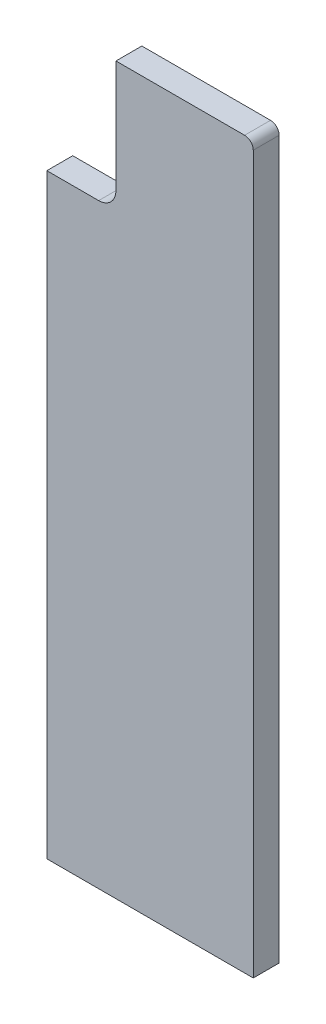
from build123d import *

# Parameters (mm, degrees)
BOSS_EXTRUDE1_DEPTH = 30
FILLET1_R           = 10


with BuildPart() as part:
    # Sketch1 → Boss-Extrude1 (new body)
    with BuildSketch(Plane.XY):
        with BuildLine():
            Line((0, 0), (239, 0))
            Line((239, 0), (239, 840))
            Line((239, 840), (80, 840))
            Line((80, 840), (80, 710))
            ThreePointArc((80, 710), (74.142135624, 695.857864376), (60, 690))
            Line((60, 690), (0, 690))
            Line((0, 690), (0, 0))
        make_face()
    extrude(amount=BOSS_EXTRUDE1_DEPTH)

    # Fillet1
    fillet1_edges = [part.edges().sort_by_distance(p)[0] for p in [
        (239, 840, 15),
    ]]
    fillet(fillet1_edges, radius=FILLET1_R)


solid = part.part
